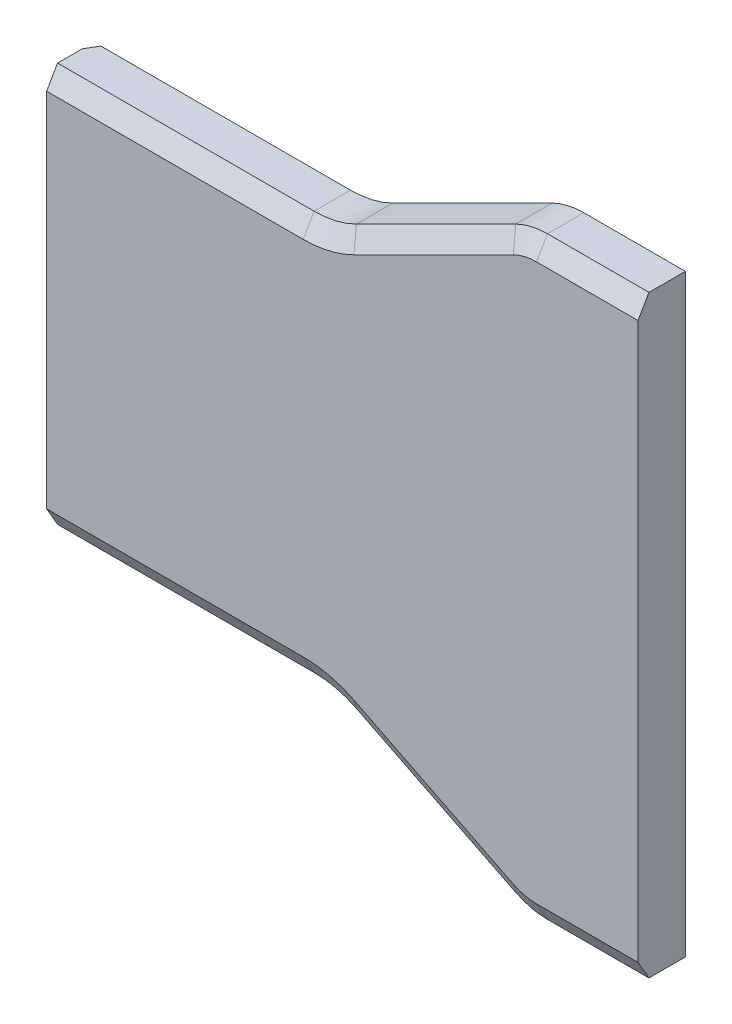
from build123d import *

# Parameters (mm, degrees)
EXTRUDE_1_DEPTH = 20
CHAMFER_1_SIZE  = 8
CHAMFER_1_SIZE2 = 4.618802154
CHAMFER_3_SIZE  = 5
CHAMFER_3_SIZE2 = 2.886751346


with BuildPart() as part:
    # 草图1 → 凸台-拉伸1 (new body)
    with BuildSketch(Plane.XY):
        with BuildLine():
            Line((-305.507868128, -251), (-322.917960675, -251))
            ThreePointArc((-322.917960675, -251), (-329.810548291, -250.197469684), (-336.33436854, -247.83281573))
            Line((-336.33436854, -247.83281573), (-403.66563146, -214.16718427))
            ThreePointArc((-403.66563146, -214.16718427), (-412.364058458, -211.014312331), (-421.55417528, -209.94427191))
            Line((-421.55417528, -209.94427191), (-530, -209.94427191))
            Line((-530, -209.94427191), (-530, -41.05572809))
            Line((-530, -41.05572809), (-421.55417528, -41.05572809))
            ThreePointArc((-421.55417528, -41.05572809), (-412.364058458, -39.985687669), (-403.66563146, -36.83281573))
            Line((-403.66563146, -36.83281573), (-336.33436854, -3.16718427))
            ThreePointArc((-336.33436854, -3.16718427), (-329.810548291, -0.802530316), (-322.917960675, 0))
            Line((-322.917960675, 0), (-300, 0))
            Line((-300, 0), (-280, 0))
            Line((-280, 0), (-280, -251))
            Line((-280, -251), (-305.507868128, -251))
        make_face()
    extrude(amount=-EXTRUDE_1_DEPTH)

    # 倒角1
    chamfer_1_edges = [part.edges().sort_by_distance(p)[0] for p in [
        (-301.458980338, -251, 0),
        (-329.810548291, -250.197469684, 0),
        (-370, -231, 0),
        (-412.364058458, -211.014312331, 0),
        (-475.77708764, -209.94427191, 0),
        (-475.77708764, -41.05572809, 0),
        (-412.364058458, -39.985687669, 0),
        (-370, -20, 0),
        (-329.810548291, -0.802530316, 0),
        (-301.458980338, 0, 0),
    ]]
    chamfer_1_side = [part.faces().sort_by_distance(p)[0] for p in [
        (-393.523242802, -125.5, 0),
    ]]
    chamfer(chamfer_1_edges, length=CHAMFER_1_SIZE, length2=CHAMFER_1_SIZE2, reference=chamfer_1_side[0])

    # 倒角3
    chamfer_3_edges = [part.edges().sort_by_distance(p)[0] for p in [
        (-530, -125.5, -20),
    ]]
    chamfer_3_side = [part.faces().sort_by_distance(p)[0] for p in [
        (-530, -125.5, -10.093574404),
    ]]
    chamfer(chamfer_3_edges, length=CHAMFER_3_SIZE, length2=CHAMFER_3_SIZE2, reference=chamfer_3_side[0])


solid = part.part
